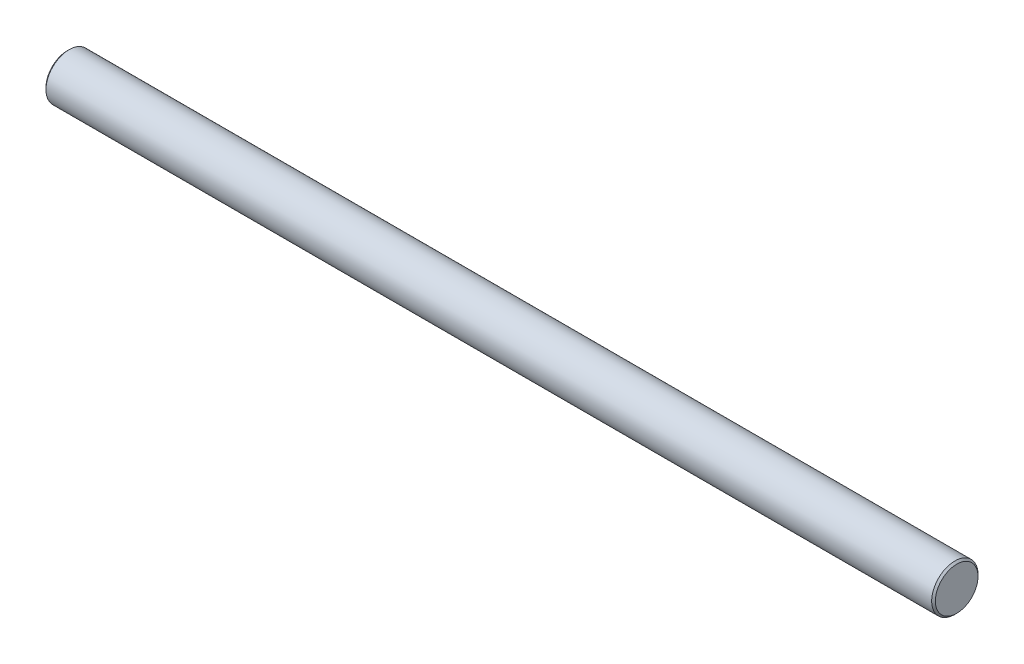
SolidWorks part; units mm, degrees
material "S45C"
ref_plane "Front Plane" through (0, 0, 0) normal (0, 0, 1) x (1, 0, 0)
ref_plane "Top Plane" through (0, 0, 0) normal (0, 1, 0) x (1, 0, 0)
ref_plane "Right Plane" through (0, 0, 0) normal (1, 0, 0) x (0, 0, -1)
sketch "Sketch1" plane through (0, 0, 0) normal (1, 0, 0) x (0, 0, -1)
  circle A0 centre (0, 0) radius 12.5
  dimension "D1" = 25
extrude "Boss-Extrude1" add sketch "Sketch1" along normal blind 480
chamfer "Chamfer1" distance 1 angle 45 2 edges at (480, 0, -12.5) (0, 0, -12.5)
